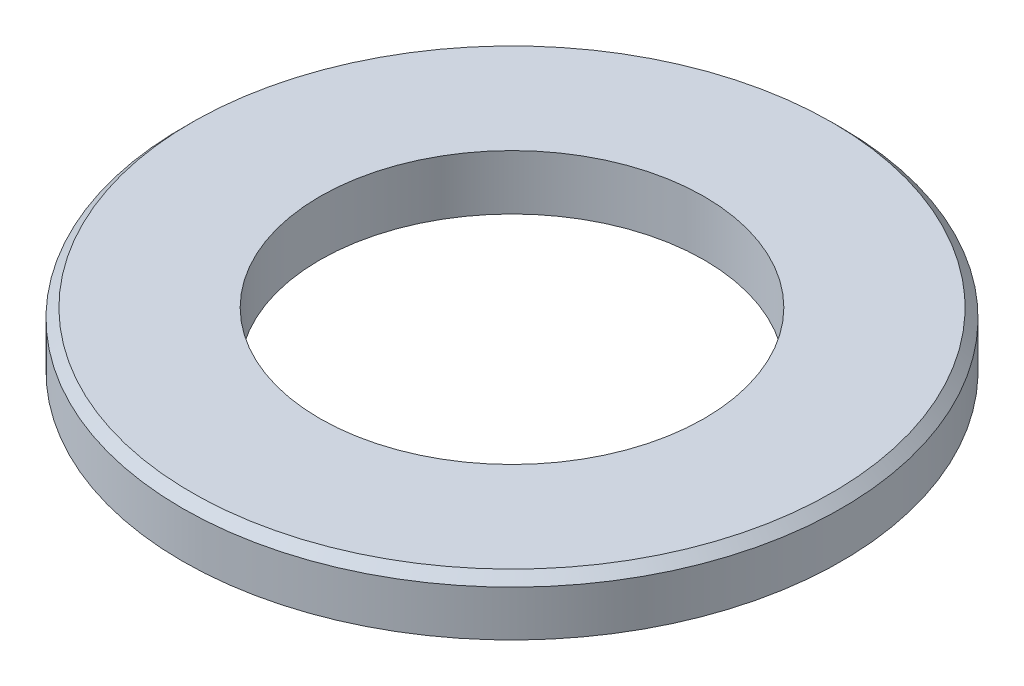
from build123d import *


with BuildPart() as part:
    # Sketch1 → Base-Revolve (revolve)
    with BuildSketch(Plane.XY, mode=Mode.PRIVATE) as base_revolve_sk:
        Polygon((-35, 14.644507042), (-36, 13.644507042), (-36, 8.644507042), (-21, 8.644507042), (-21, 14.644507042), align=None)
    revolve(base_revolve_sk.sketch.rotate(Axis((0, 0, 0), (0, 1, 0)), 270), axis=Axis((0, 0, 0), (0, 1, 0)))


solid = part.part
